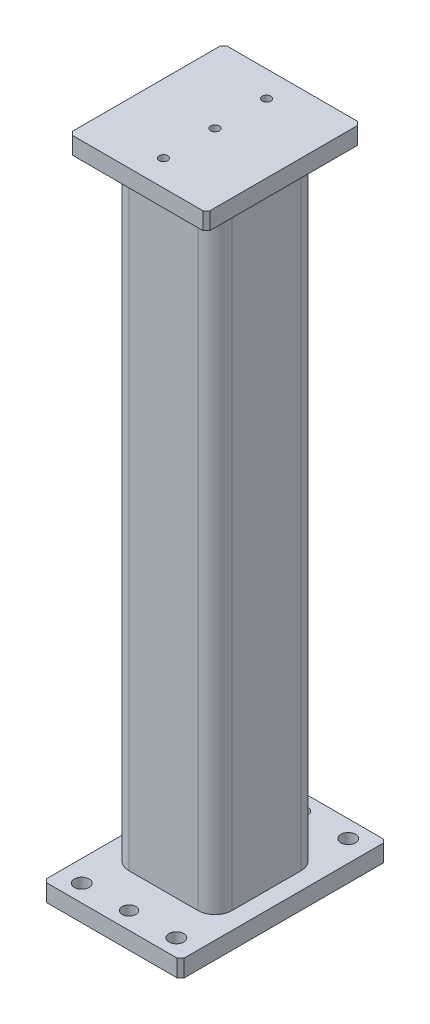
from build123d import *

# Parameters (mm, degrees)
MEMBER_1_DEPTH                   = 359
SKETCH_4_W                       = 80
SKETCH_4_H                       = 120
EXTRUDE_1_DEPTH                  = 10
CHAMFER_1_SIZE                   = 2
HOLE_WIZARD_8_6_8_6_1_AT_2_COUNT = 2
HOLE_WIZARD_8_6_8_6_1_AT_2_PITCH = 114.127122105
HOLE_WIZARD_8_6_8_6_1_AT_3_COUNT = 2
HOLE_WIZARD_8_6_8_6_1_AT_3_PITCH = 55
HOLE_WIZARD_8_6_8_6_1_AT_4_COUNT = 2
HOLE_WIZARD_8_6_8_6_1_AT_4_PITCH = 100
HOLE_WIZARD_8_0_8_1_AT_2_COUNT   = 2
HOLE_WIZARD_8_0_8_1_AT_2_PITCH   = 100
SKETCH_13_W                      = 80
SKETCH_13_H                      = 90
EXTRUDE_2_DEPTH                  = 10
CHAMFER_2_SIZE                   = 2
HOLE_WIZARD_M6_1_AT_2_COUNT      = 2
HOLE_WIZARD_M6_1_AT_2_PITCH      = 60


with BuildPart() as part:
    # Sketch1 → Member 1 (new body)
    with BuildSketch(Plane(origin=(0, 0, 0), x_dir=(-1, 0, 0), z_dir=(0, 1, 0))):
        with BuildLine():
            Line((-20, -30), (20, -30))
            ThreePointArc((20, -30), (27.071067812, -27.071067812), (30, -20))
            Line((30, -20), (30, 20))
            ThreePointArc((30, 20), (27.071067812, 27.071067812), (20, 30))
            Line((20, 30), (-20, 30))
            ThreePointArc((-20, 30), (-27.071067812, 27.071067812), (-30, 20))
            Line((-30, 20), (-30, -20))
            ThreePointArc((-30, -20), (-27.071067812, -27.071067812), (-20, -30))
        make_face()
        with BuildLine():
            Line((-20, -25), (20, -25))
            ThreePointArc((20, -25), (23.535533906, -23.535533906), (25, -20))
            Line((25, -20), (25, 20))
            ThreePointArc((25, 20), (23.535533906, 23.535533906), (20, 25))
            Line((20, 25), (-20, 25))
            ThreePointArc((-20, 25), (-23.535533906, 23.535533906), (-25, 20))
            Line((-25, 20), (-25, -20))
            ThreePointArc((-25, -20), (-23.535533906, -23.535533906), (-20, -25))
        make_face(mode=Mode.SUBTRACT)
    extrude(amount=MEMBER_1_DEPTH)


with BuildPart() as body_2:
    # 草图4 → 凸台-拉伸1 (new body)
    with BuildSketch(Plane.XZ):
        Rectangle(SKETCH_4_W, SKETCH_4_H)
    extrude(amount=EXTRUDE_1_DEPTH)

    # 倒角1
    chamfer_1_edges = [body_2.edges().sort_by_distance(p)[0] for p in [
        (40, -5, -60),
        (-40, -5, -60),
        (-40, -5, 60),
        (40, -5, 60),
    ]]
    chamfer(chamfer_1_edges, length=CHAMFER_1_SIZE)

    # 草图5 → Ø8.6 (8.6) 直径孔1 (revolve, cut)
    with BuildSketch(Plane(origin=(27.5, 0, -50), x_dir=(0, 0, 1), z_dir=(1, 0, 0))):
        Polygon((0, 0), (0, 18.092606158), (4.3, 15.61), (4.3, 0), align=None)
    hole_wizard_8_6_8_6_1 = revolve(axis=Axis((27.5, 6.35, -50), (0, -1, 0)), mode=Mode.SUBTRACT)

    # Ø8.6 (8.6) 直径孔1 at 2: Ø8.6 (8.6) 直径孔1 ×2
    with Locations(*[Vector(-0.481918749772156, 0, 0.876215908676647) * (i * HOLE_WIZARD_8_6_8_6_1_AT_2_PITCH) for i in range(1, HOLE_WIZARD_8_6_8_6_1_AT_2_COUNT)]):
        add(hole_wizard_8_6_8_6_1, mode=Mode.SUBTRACT)

    # Ø8.6 (8.6) 直径孔1 at 3: Ø8.6 (8.6) 直径孔1 ×2
    with Locations(*[(-i * HOLE_WIZARD_8_6_8_6_1_AT_3_PITCH, 0, 0) for i in range(1, HOLE_WIZARD_8_6_8_6_1_AT_3_COUNT)]):
        add(hole_wizard_8_6_8_6_1, mode=Mode.SUBTRACT)

    # Ø8.6 (8.6) 直径孔1 at 4: Ø8.6 (8.6) 直径孔1 ×2
    with Locations(*[(0, 0, i * HOLE_WIZARD_8_6_8_6_1_AT_4_PITCH) for i in range(1, HOLE_WIZARD_8_6_8_6_1_AT_4_COUNT)]):
        add(hole_wizard_8_6_8_6_1, mode=Mode.SUBTRACT)

    # 草图11 → Ø8.0 (8) 直径孔1 (revolve, cut)
    with BuildSketch(Plane(origin=(0, 0, -50), x_dir=(0, 0, 1), z_dir=(1, 0, 0))):
        Polygon((0, 0), (0, 17.919401077), (4, 15.61), (4, 0), align=None)
    hole_wizard_8_0_8_1 = revolve(axis=Axis((0, 6.35, -50), (0, -1, 0)), mode=Mode.SUBTRACT)

    # Ø8.0 (8) 直径孔1 at 2: Ø8.0 (8) 直径孔1 ×2
    with Locations(*[(0, 0, i * HOLE_WIZARD_8_0_8_1_AT_2_PITCH) for i in range(1, HOLE_WIZARD_8_0_8_1_AT_2_COUNT)]):
        add(hole_wizard_8_0_8_1, mode=Mode.SUBTRACT)


with BuildPart() as body_3:
    # 草图13 → 凸台-拉伸2 (new body)
    with BuildSketch(Plane(origin=(0, 359, 0), x_dir=(1, 0, 0), z_dir=(0, 1, 0))):
        Rectangle(SKETCH_13_W, SKETCH_13_H)
    extrude(amount=EXTRUDE_2_DEPTH)

    # 倒角2
    chamfer_2_edges = [body_3.edges().sort_by_distance(p)[0] for p in [
        (40, 364, 45),
        (-40, 364, 45),
        (-40, 364, -45),
        (40, 364, -45),
    ]]
    chamfer(chamfer_2_edges, length=CHAMFER_2_SIZE)

    # 草图15 → Ø5.0 (5) 直径孔1 (revolve, cut)
    with BuildSketch(Plane(origin=(0, 369, 0), x_dir=(0, 0, 1), z_dir=(1, 0, 0))):
        Polygon((0, 0), (0, 17.053375673), (2.5, 15.61), (2.5, 0), align=None)
    revolve(axis=Axis((0, 375.35, 0), (0, -1, 0)), mode=Mode.SUBTRACT)

    # 草图17 → M6 螺纹孔1 (revolve, cut)
    with BuildSketch(Plane(origin=(0, 369, -30), x_dir=(0, 0, 1), z_dir=(1, 0, 0))):
        Polygon((0, 0), (0, 18.502151548), (2.5, 17), (2.5, 0), align=None)
    hole_wizard_m6_1 = revolve(axis=Axis((0, 375.35, -30), (0, -1, 0)), mode=Mode.SUBTRACT)

    # M6 螺纹孔1 at 2: M6 螺纹孔1 ×2
    with Locations(*[(0, 0, i * HOLE_WIZARD_M6_1_AT_2_PITCH) for i in range(1, HOLE_WIZARD_M6_1_AT_2_COUNT)]):
        add(hole_wizard_m6_1, mode=Mode.SUBTRACT)


solid = Compound([part.part, body_2.part, body_3.part])
